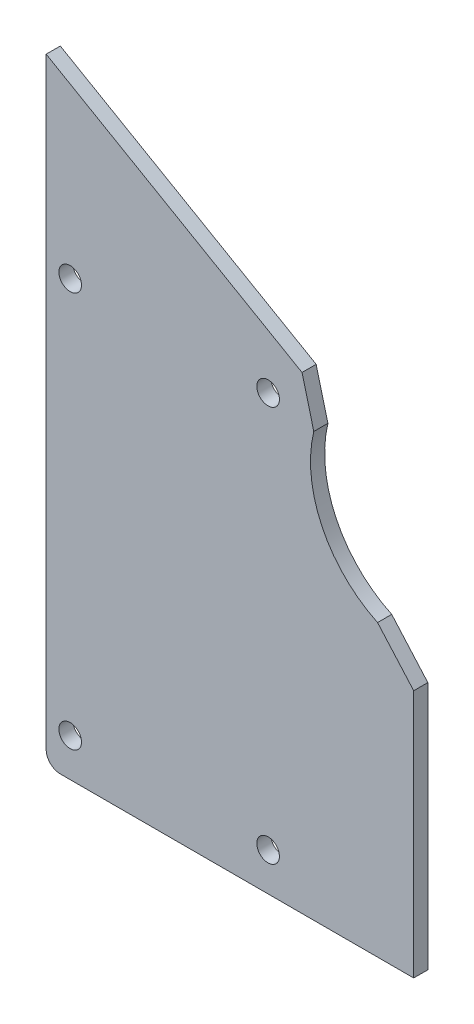
from build123d import *

# Parameters (mm, degrees)
BOSS_EXTRUDE1_DEPTH        = 5
F_16_0_16_DIAMETER_HOLE1_D = 16
FILLET1_R                  = 10


with BuildPart() as part:
    # Sketch1 → Boss-Extrude1 (new, symmetric)
    with BuildSketch(Plane.XY):
        with BuildLine():
            Line((0, 0), (0, 436))
            Line((0, 436), (181, 331.499601277))
            Line((181, 331.499601277), (189.323079198, 299.499601277))
            ThreePointArc((189.323079198, 299.499601277), (195.100872088, 244.235203929), (234.447222331, 205))
            Line((234.447222331, 205), (260, 176))
            Line((260, 176), (260, 0))
            Line((260, 0), (0, 0))
        make_face()
    extrude(amount=BOSS_EXTRUDE1_DEPTH, both=True)

    # Ø16.0 (16) Diameter Hole1 (through all)
    with Locations(Plane.XY.offset(5)):
        with Locations((17, 27), (157, 27), (157, 307), (17, 307)):
            Hole(F_16_0_16_DIAMETER_HOLE1_D / 2)

    # Fillet1
    fillet1_edges = [part.edges().sort_by_distance(p)[0] for p in [
        (0, 0, 0),
    ]]
    fillet(fillet1_edges, radius=FILLET1_R)


solid = part.part
